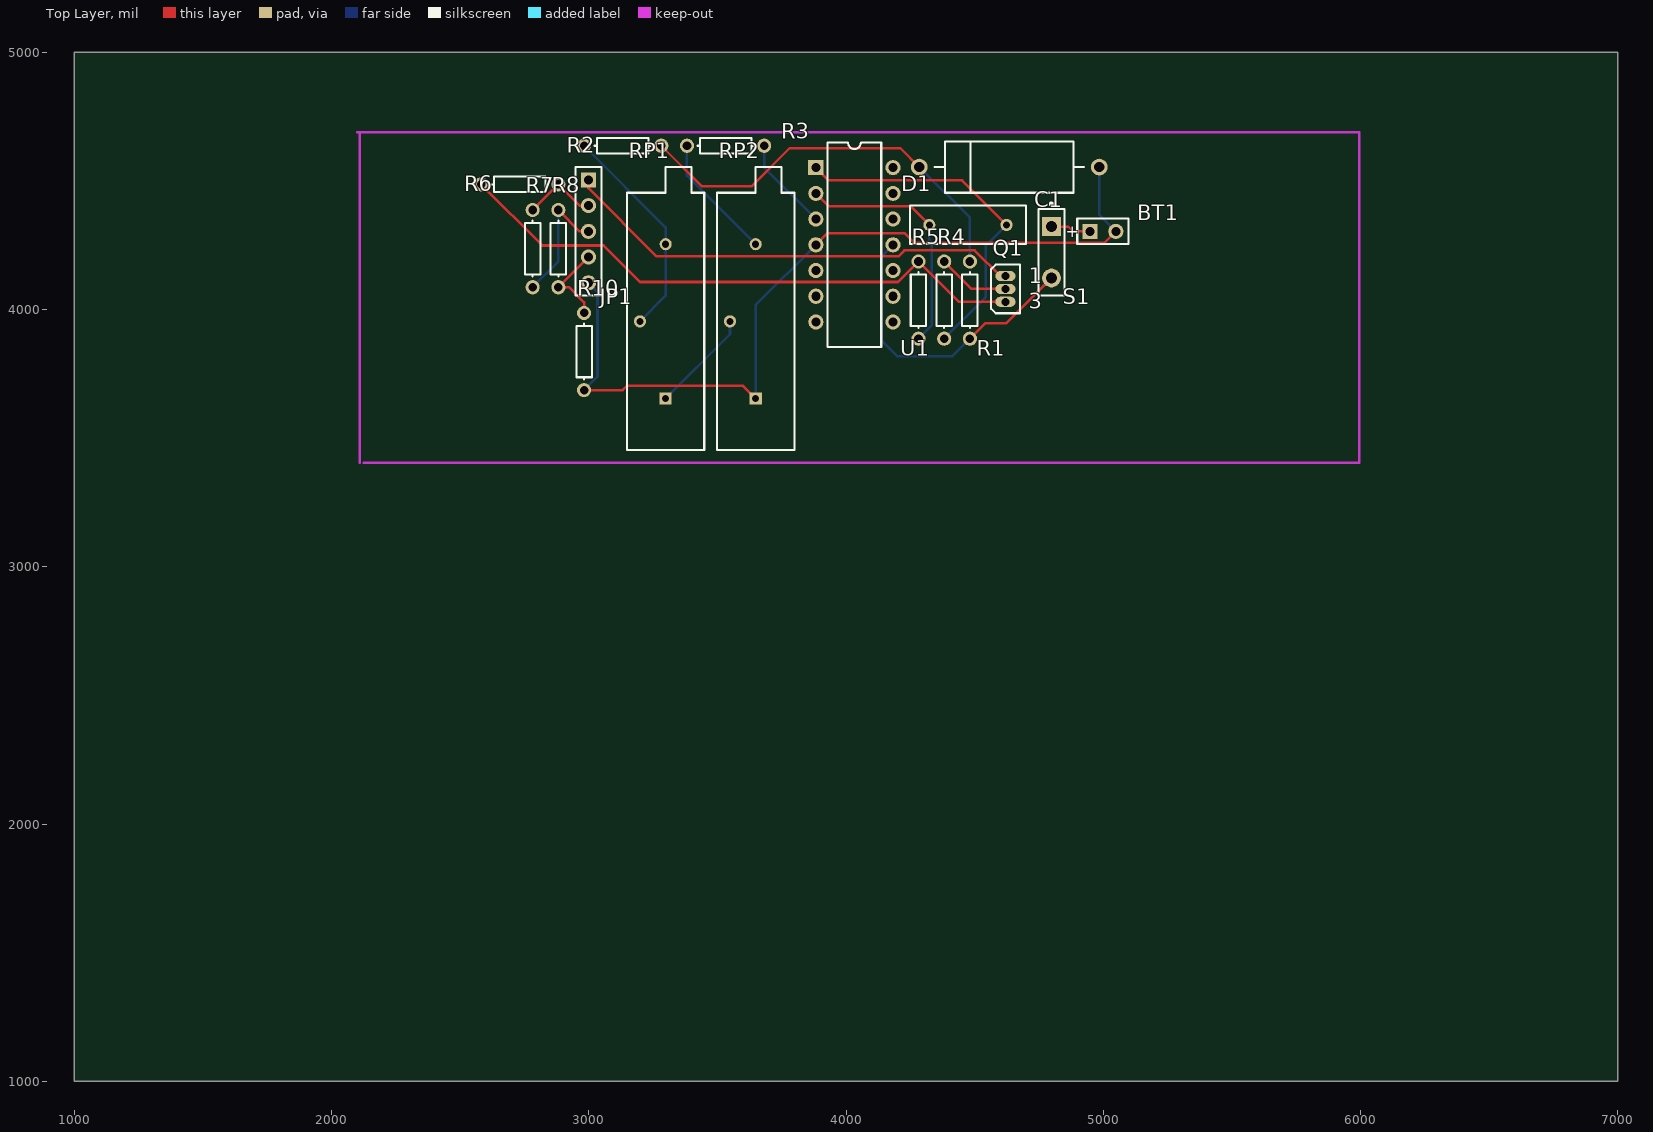
[diagram p0: Top Layer view]
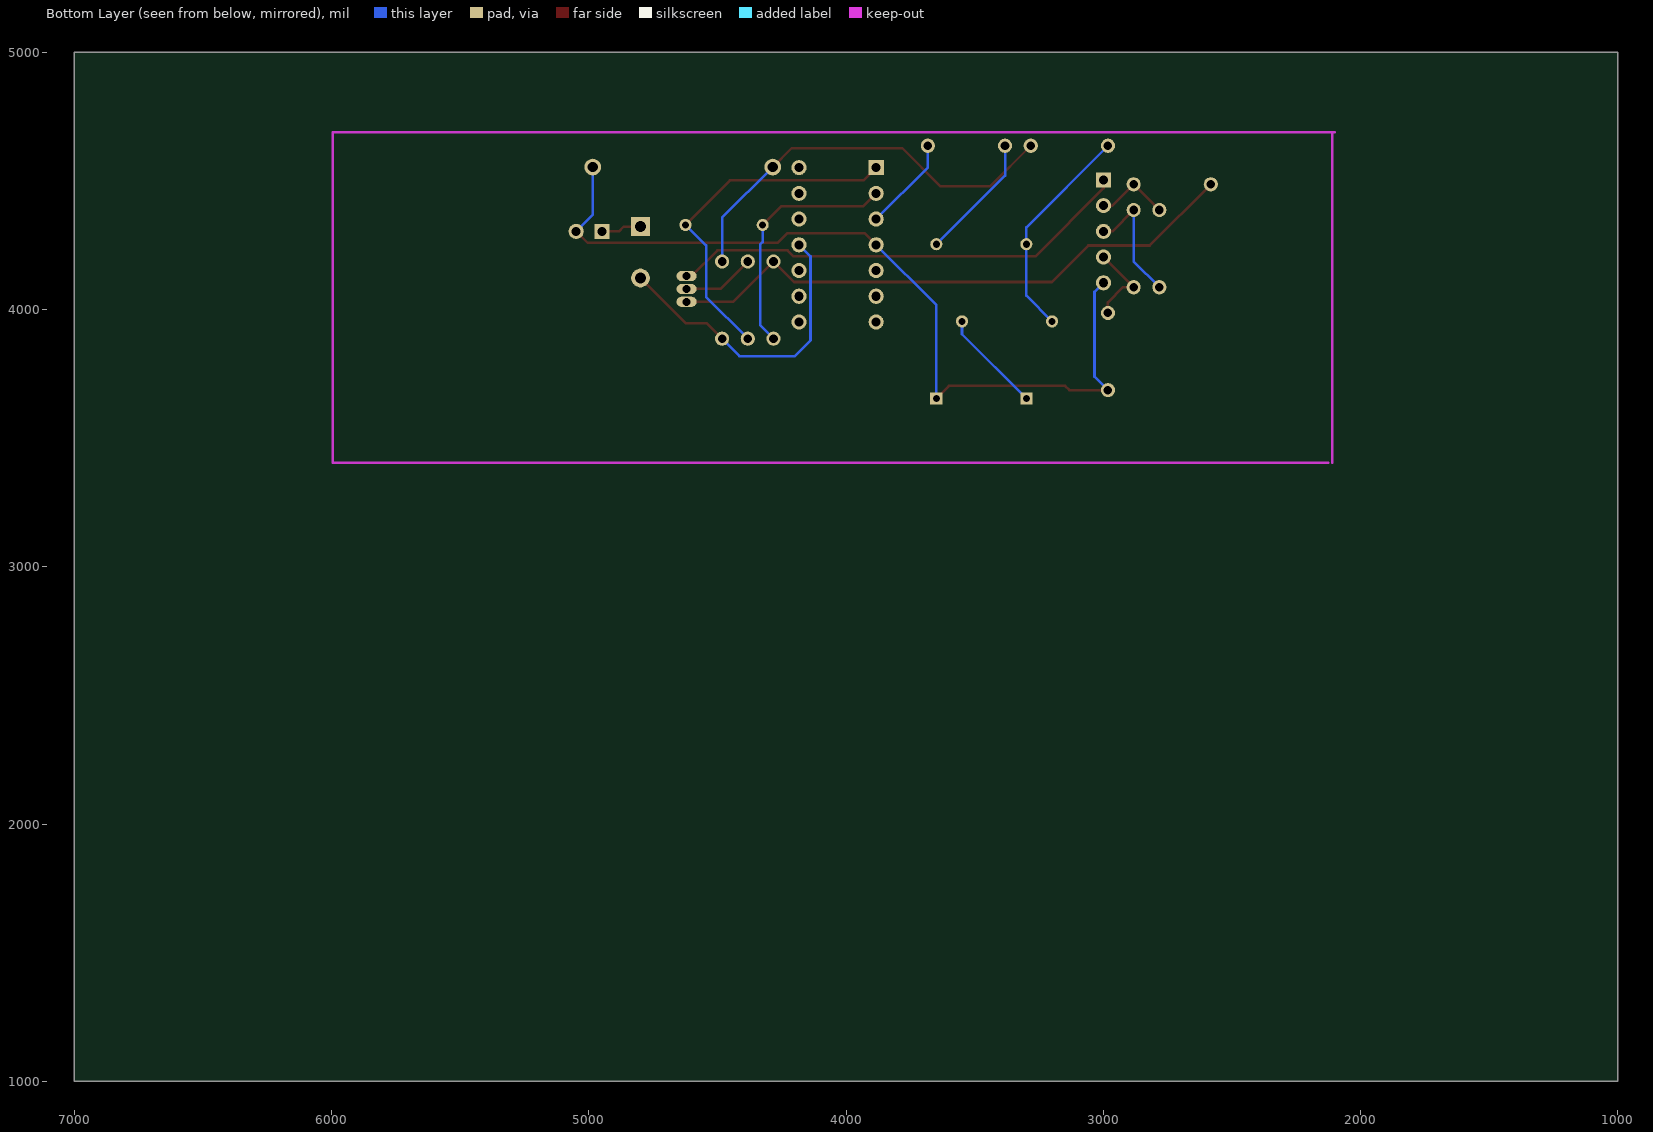
[diagram p1: Bottom Layer view, seen from below]
# Altium PCB MISC95142.PCBDOC
Units mil, origin at the board's own origin, x right, y up, seen from the top; angles counter-clockwise.
Board outline 6000 x 4000 mil, 2 copper layers (Top Layer, Bottom Layer); 18 components, 16 nets, 54 pads, 0 vias.

## Layer stack, top to bottom (the 12.6 mil dielectric is the usual default, probably not edited)
Top Layer: signal copper 1.4
Dielectric: dielectric 12.6, FR-4, Dk 4.8
Bottom Layer: signal copper 1.4

## Board outline
1000,1000 7000,1000 7000,5000 1000,5000

## Design rules (kind name [scope] priority, off if disabled: settings)
Clearance [All] p1: gap=10
ComponentClearance [All] p1: gap=10 collisioncheckmode=0
PolygonConnect [All] p1: connectstyle=Relief reliefconductorwidth=10 reliefentries=4 polygonreliefangle="90 Angle"
RoutingLayers [All] p1: top layer=Horizontal bottom layer=Vertical
RoutingVias [All] p1: holewidth=28 width=50 viastyle="Through Hole" minholewidth=28 minwidth=50 maxholewidth=28 maxwidth=50
SolderMaskExpansion [All] p1: expansion=4
TestPointUsage [All] p1: valid=0 allowmultiple=FALSE
Testpoint [All] p1: side=15 testpointundercomponent=TRUE minsize=40 maxsize=100 preferedsize=60 minholesize=0 maxholesize=40 preferedholesize=32 testpointgrid=1 style=1023 order=1234567890
Width [All] p1: maxlimit=10 minlimit=10 preferedwidth=10
16 further rules are at their usual default settings.

## Components (designator, comment, footprint, x,y, rotation, side; value= is the part's Value field where it differs from the comment)
BT1 "Battery" BAT-2 4998.94,4303.94 r0 top
C1 "Cap" RAD-0.3 4473.94,4328.94 r0 top
D1 "D Zener" DIODE-0.7 4634.69,4553.94 r180 top
JP1 "Header 5" HDR1X5 2998.94,4503.94 r270 top
Q1 "MOSFET-N" BCY-W3/H.8 4620,4080 r0 top
R1 "Res1" AXIAL-0.3 4481.73,4036.73 r270 top
R2 "Res1" AXIAL-0.3 3131.73,4636.73 r180 top
R3 "Res1" AXIAL-0.3 3531.73,4636.73 r0 top
R4 "Res1" AXIAL-0.3 4381.73,4036.73 r90 top
R5 "Res1" AXIAL-0.3 4281.73,4036.73 r90 top
R6 "Res1" AXIAL-0.3 2731.73,4486.73 r180 top
R7 "Res1" AXIAL-0.3 2781.73,4236.73 r90 top
R8 "Res1" AXIAL-0.3 2881.73,4236.73 r90 top
R10 "Res1" AXIAL-0.3 2981.73,3836.73 r90 top
RP1 "RPot" VR2 3248.94,3953.94 r90 top
RP2 "RPot" VR2 3598.94,3953.94 r90 top
S1 "SW-SPST" SPST-2 4798.94,4222.44 r270 top
U1 "LM248J" J014 4032.72,4251.57 r270 top

## Footprints (in the part's own frame and the unit in brackets; to place one, negate y for a bottom-side part, rotate by r counter-clockwise, add the part's x,y. Pads: shape width x height; smd on the part's side, far side on the other; paste and mask are expansions set on the pad)
AXIAL-0.3 [mm]
  round 1.4 hole 0.85: 1(-3.81,0) 2(3.81,0)
  silkscreen extent -2.77,-0.76 2.77,0.76
BAT-2 [mm]
  rect 1.5x1.5 hole 0.9: 1(-1.27,0)
  round 1.5 hole 0.9: 2(1.27,0)
  silkscreen extent -2.54,-1.27 2.54,1.27
BCY-W3/H.8 [mm]
  oval 2x1 hole 0.8: 1(0,1.27) 2(0,0) 3(0,-1.27)
  silkscreen extent -1.41,-2.41 1.41,2.41
DIODE-0.7 [mm]
  round 1.65 hole 1: 1(-8.89,0) 2(8.89,0)
  silkscreen extent -7.37,-2.54 7.37,2.54
HDR1X5 [mm] "Connector; Header; 5 Position"
  rect 1.5x1.5 hole 0.9: 1(0,0)
  round 1.5 hole 0.9: 2(2.54,0) 3(5.08,0) 4(7.62,0) 5(10.16,0)
  silkscreen extent -1.27,-1.27 11.43,1.27
J014 [mm] "DIP; 14 Leads; Row Spacing 7.62 mm; Pitch 2.54 mm"
  rect 1.5x1.5 hole 0.9: 1(-7.62,-3.81)
  round 1.5 hole 0.9: 2(-5.08,-3.81) 3(-2.54,-3.81) 4(0,-3.81) 5(2.54,-3.81) 6(5.08,-3.81) 7(7.62,-3.81) 8(7.62,3.81) 9(5.08,3.81) 10(2.54,3.81) 11(0,3.81) 12(-2.54,3.81) 13(-5.08,3.81) 14(-7.62,3.81)
  silkscreen extent -10.1,-2.65 10.1,2.65
RAD-0.3 [mm]
  round 1.2 hole 0.7: 1(-3.81,0) 2(3.81,0)
  silkscreen extent -5.71,-1.9 5.72,1.91
SPST-2 [mm]
  rect 1.85x1.85 hole 1.1: 1(-2.54,0)
  round 1.85 hole 1.1: 2(2.54,0)
  silkscreen extent -4.89,-1.27 4.28,1.27
VR2 [mm]
  rect 1.2x1.2 hole 0.7: 1(-7.62,-1.27)
  round 1.2 hole 0.7: 2(0,1.27) 3(7.62,-1.27)
  silkscreen extent -12.7,-5.08 15.24,2.54

## Part data
BT1: "Multicell Battery"
C1: "Capacitor"
D1: "Zener Diode"
JP1: "Header, 5-Pin"
Q1: "N-Channel MOSFET"
R1 R2 R3 R4 R5 R6 R7 R8 R10: "Resistor"
RP1 RP2: "Potentiometer"
S1: "Single-Pole, Single-Throw Switch"
U1: "Quadruple Operational Amplifier"

## Nets (pads, with @x,y where several pads share a name; then routed paths per layer and width w, separated by ;. In a path a pad name is that pad's centre, name@x,y a point inside that pad or via, vN(x,y) a via of type N, cw(c..) or ccw(c..) an arc to the next point about the centre after c; other vN are vias at no path point)
GND: BT1.2 D1.1 JP1.5 R10.1 RP2.1 U1.4 | length 3338.1
  Top Layer w10: R10.1 3132,3686.73 3148.27,3703 3599.88,3703 RP2.1 ; U1.4 3928.14,4297 4228,4297 4266,4259 5004,4259 BT1.2
  Bottom Layer w10: R10.1 3034,3739 3034,4068.88 JP1.5 ; RP2.1 3648.94,4017.8 U1.4 ; D1.1 4984.69,4368.19 BT1.2
NetBT1_1: BT1.1 S1.1 | length 157.7
  Top Layer w10: S1.1 4864,4322.44 4882.5,4303.94 BT1.1
NetC1_1: C1.1 R5.1 U1.2 | length 960
  Top Layer w10: U1.2 3932.29,4402 4250.88,4402 C1.1
  Bottom Layer w10: R5.1 4334,3939 4334,4251.94 4323.94,4262 C1.1
NetC1_2: C1.2 R4.1 U1.1 | length 1376
  Top Layer w10: U1.1 3932.29,4502 4450.88,4502 C1.2
  Bottom Layer w10: R4.1 4544,4049 4544,4249 C1.2
NetD1_2: D1.2 R1.1 R2.1 | length 1607.9
  Top Layer w10: R2.1 3438.46,4480 3634,4480 3781,4627 4211.62,4627 D1.2
  Bottom Layer w10: D1.2 4481.73,4356.89 R1.1
NetJP1_1: JP1.1 Q1.1 | length 1813.7
  Top Layer w10: JP1.1 2998.94,4472.06 3264,4207 4204,4207 4227,4230 4500,4230 4600,4130 Q1.1
NetJP1_2: JP1.2 R6.1 R7.2 | length 293.4
  Top Layer w10: R7.2 2781.73,4387.46 2881,4486.73 R6.1 2964.53,4403.94 JP1.2
NetJP1_3: JP1.3 R7.1 R8.2 | length 492.9
  Top Layer w10: R8.2 2964.53,4303.94 JP1.3
  Bottom Layer w10: R7.1 2881.73,4186.73 R8.2
NetJP1_4: JP1.4 R8.1 R10.2 | length 330.9
  Top Layer w10: R10.2 2981.73,4027.27 2922.27,4086.73 R8.1 JP1.4
NetQ1_2: Q1.2 R4.2 | length 282.5
  Top Layer w10: R4.2 4488.46,4080 Q1.2
NetQ1_3: Q1.3 R5.2 R6.2 | length 2293.5
  Top Layer w10: R6.2 2819.46,4249 3058,4249 3200,4107 4202,4107 R5.2 4438.46,4030 Q1.3
NetR1_2: R1.2 S1.2 U1.11 | length 1202
  Top Layer w10: R1.2 4541,3946 4622.5,3946 S1.2
  Bottom Layer w10: U1.11 4138,4206.86 4138,3880 4199,3819 4414,3819 R1.2
NetR2_2: R2.2 RP1.2 RP1.3 | length 855.6
  Bottom Layer w10: R2.2 3298.94,4319.53 RP1.3 3298.94,4053.94 RP1.2
NetR3_1: R3.1 RP2.3 | length 493.5
  Bottom Layer w10: R3.1 3381.73,4521.14 RP2.3
NetR3_2: R3.2 U1.3 | length 368.4
  Bottom Layer w10: R3.2 3681.73,4552.56 U1.3
NetRP1_1: RP1.1 RP2.2 | length 403.6
  Bottom Layer w10: RP1.1 3548.94,3903.94 RP2.2
pads on no net: U1.5 U1.6 U1.7 U1.8 U1.9 U1.10 U1.12 U1.13 U1.14

## Keep-outs
Keep-Out Layer:
  lines w10: 2100,4690 5995,4690 5995,3405 2125,3405 ; 2110,3405 2110,4690